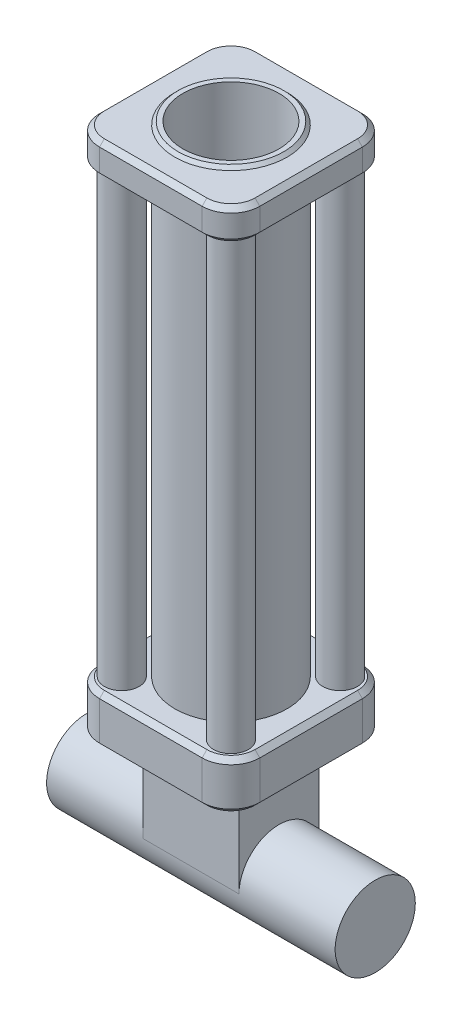
SolidWorks part; units mm, degrees
ref_plane "Front Plane" through (0, 0, 0) normal (0, 0, 1) x (1, 0, 0)
ref_plane "Top Plane" through (0, 0, 0) normal (0, 1, 0) x (1, 0, 0)
ref_plane "Right Plane" through (0, 0, 0) normal (1, 0, 0) x (0, 0, -1)
sketch "Sketch1" plane through (0, 0, 0) normal (0, 1, 0) x (1, 0, 0)
  circle A0 centre (0, 0) radius 175
  circle A1 centre (0, 0) radius 150
  dimension "D1" = 350
  dimension "D2" = 300
extrude "Boss-Extrude1" add sketch "Sketch1" along normal blind 1500
sketch "Sketch2" plane through (0, 0, 0) normal (0, -1, 0) x (1, 0, 0)
  line L1 (-250, 250) -> (250, 250)
  line L2 (-250, 250) -> (-250, -250)
  line L3 (-250, -250) -> (250, -250)
  line L4 (250, 250) -> (250, -250)
  line L5 (-250, 250) -> (250, -250) construction
  line L6 (-250, -250) -> (250, 250) construction
  point P0 (0, 0)
  dimension "D1" = 500
  dimension "D2" = 500
extrude "Boss-Extrude2" add sketch "Sketch2" along normal blind 150
sketch "Sketch3" plane through (0, 0, 0) normal (1, 0, 0) x (0, 0, -1)
  line L0 (0, -150) -> (0, -450) construction
  line L1 (0, 275) -> (0, -275) construction
  line L2 (125, -150) -> (125, -450)
  line L3 (-125, -150) -> (-125, -450)
  line L4 (-125, -150) -> (125, -150)
  arc A1 (-125, -450) -> (125, -450) centre (0, -450) ccw
  point P5 (0, -300)
  dimension "D2" = 125
  dimension "D1" = 300
extrude "Boss-Extrude3" add sketch "Sketch3" along normal blind 150 and the other way blind 150
sketch "Sketch4" plane through (0, 0, 0) normal (1, 0, 0) x (0, 0, -1)
  circle A0 centre (0, -450) radius 125
extrude "Boss-Extrude4" add sketch "Sketch4" along normal blind 450 and the other way blind 450
chamfer "Chamfer2" distance 10 angle 45 1 edges at (0, 1500, 175)
ref_plane "Plane1" through (0, 1490, 0) normal (0, 1, 0) x (1, 0, 0)
sketch "Sketch5" plane through (0, 1490, 0) normal (0, 1, 0) x (1, 0, 0)
  line L1 (-250, 250) -> (250, 250)
  line L2 (-250, 250) -> (-250, -250)
  line L3 (-250, -250) -> (250, -250)
  line L4 (250, 250) -> (250, -250)
  line L5 (-250, 250) -> (250, -250) construction
  line L6 (-250, -250) -> (250, 250) construction
  circle A0 centre (0, 0) radius 154.8875
  point P0 (0, 0)
extrude "Boss-Extrude5" add sketch "Sketch5" against normal blind 100
sketch "Sketch6" plane through (0, 0, 0) normal (0, 1, 0) x (1, 0, 0)
  line L0 (-250, 250) -> (0, 0) construction
  line L1 (-250, 250) -> (-250, -250) construction
  circle A0 centre (-170.2753, 170.2753) radius 54.2266
extrude "Boss-Extrude6" add sketch "Sketch6" along normal up to next
pattern_circular "CirPattern1" count 4 over 360 about axis through (0, 0, 0) along (0, 1, 0) of "Boss-Extrude6"
fillet "Fillet1" radius 90 8 edges at (-250, 1440, -250) (-250, 1440, 250) (250, 1440, 250) (250, 1440, -250) (250, -75, -250) (250, -75, 250) (-250, -75, 250) (-250, -75, -250)
chamfer "Chamfer3" distance 15 angle 45 32 edges at (250, -150, 0) (223.6396, -150, 223.6396) (223.6396, -150, -223.6396) (0, -150, 250) (0, -150, -250) (-223.6396, -150, 223.6396) (-223.6396, -150, -223.6396) (-250, -150, 0) (250, 0, 0) (223.6396, 0, 223.6396) (223.6396, 0, -223.6396) (0, 0, 250) (0, 0, -250) (-223.6396, 0, 223.6396) (-223.6396, 0, -223.6396) (-250, 0, 0) (250, 1490, 0) (223.6396, 1490, -223.6396) (223.6396, 1490, 223.6396) (0, 1490, -250) (0, 1490, 250) (-223.6396, 1490, -223.6396) (-223.6396, 1490, 223.6396) (-250, 1490, 0) (250, 1390, 0) (223.6396, 1390, -223.6396) (223.6396, 1390, 223.6396) (0, 1390, -250) (0, 1390, 250) (-223.6396, 1390, -223.6396) (-223.6396, 1390, 223.6396) (-250, 1390, 0)
